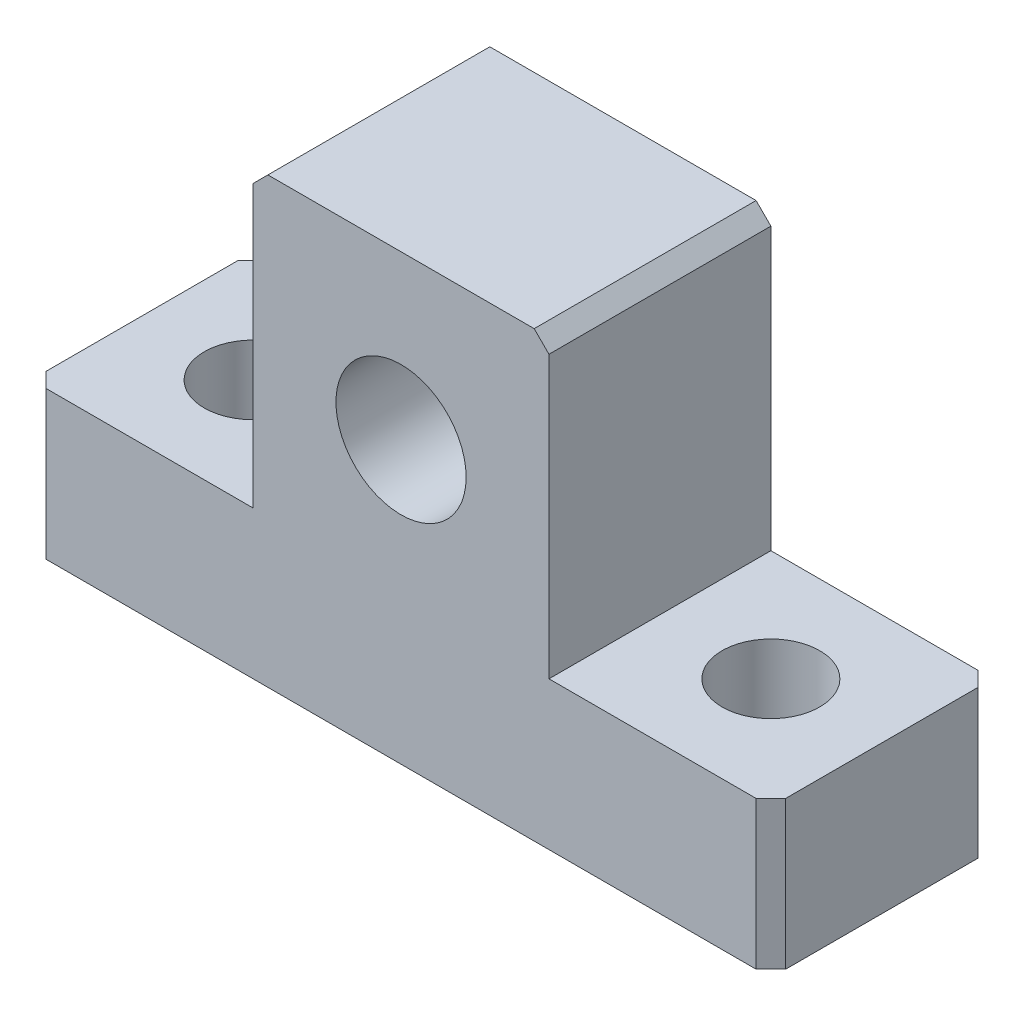
from build123d import *

# Parameters (mm, degrees)
BOSS_EXTRUDE1_DEPTH     = 15
CHAMFER1_SIZE           = 1
HOLE1_D                 = 6.6
M10X1_25_TAPPED_HOLE1_D = 8.8


with BuildPart() as part:
    # Sketch1 → Boss-Extrude1 (new body)
    with BuildSketch(Plane.XY):
        Polygon((-7.92160415, 21.721938776), (-7.92160415, 1.721938776), (-22.92160415, 1.721938776), (-22.92160415, -8.278061224), (27.07839585, -8.278061224), (27.07839585, 1.721938776), (12.07839585, 1.721938776), (12.07839585, 21.721938776), align=None)
    extrude(amount=BOSS_EXTRUDE1_DEPTH)

    # Chamfer1
    chamfer1_edges = [part.edges().sort_by_distance(p)[0] for p in [
        (-22.92160415, -3.278061224, 0),
        (12.07839585, 21.721938776, 7.5),
        (-7.92160415, 21.721938776, 7.5),
        (-22.92160415, -3.278061224, 15),
        (27.07839585, -3.278061224, 15),
        (27.07839585, -3.278061224, 0),
    ]]
    chamfer(chamfer1_edges, length=CHAMFER1_SIZE)

    # Hole1 (through all)
    with Locations(Plane(origin=(0, 1.721938776, 0), x_dir=(1, 0, 0), z_dir=(0, 1, 0))):
        with Locations((-15.42160415, -7.5), (19.57839585, -7.5)):
            Hole(HOLE1_D / 2)

    # M10x1.25 Tapped Hole1 (through all)
    with Locations(Plane.XY.offset(15)):
        with Locations((2.07839585, 10.721938776)):
            Hole(M10X1_25_TAPPED_HOLE1_D / 2)


solid = part.part
